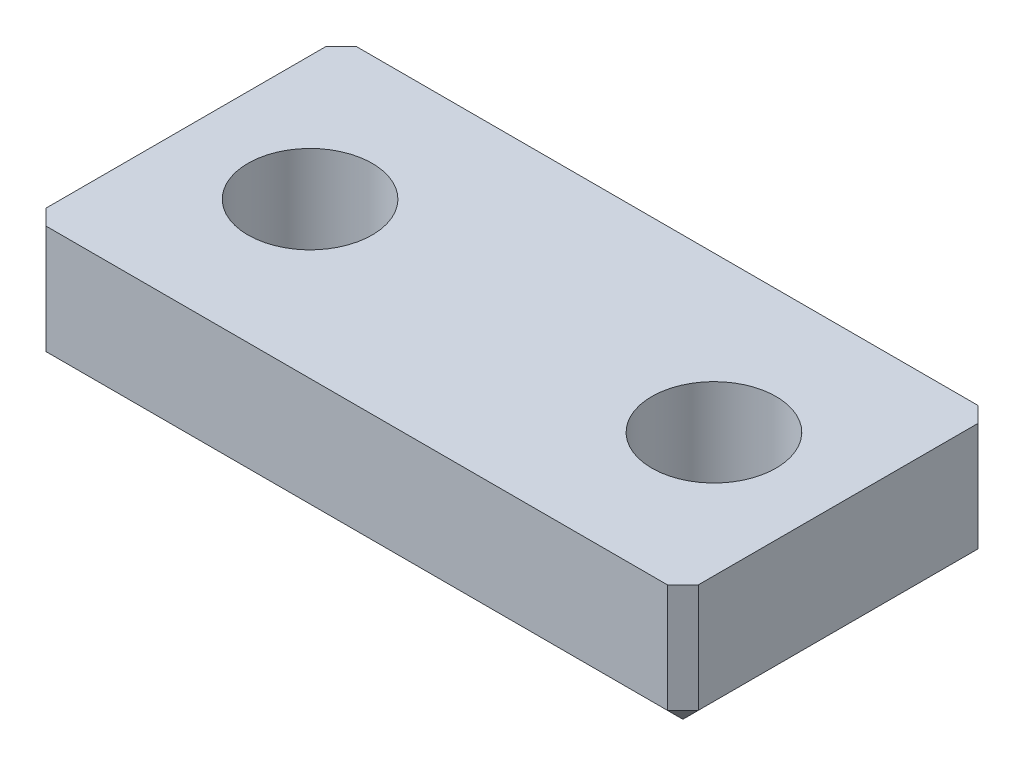
SolidWorks part; units mm, degrees
ref_plane "Front Plane" through (0, 0, 0) normal (0, 0, 1) x (1, 0, 0)
ref_plane "Top Plane" through (0, 0, 0) normal (0, 1, 0) x (1, 0, 0)
ref_plane "Right Plane" through (0, 0, 0) normal (1, 0, 0) x (0, 0, -1)
sketch "Sketch1" plane through (0, 0, 0) normal (0, 0, 1) x (1, 0, 0)
  line L1 (0, 0) -> (21, 0)
  line L2 (0, 0) -> (0, -4)
  line L3 (0, -4) -> (21, -4)
  line L4 (21, 0) -> (21, -4)
  dimension "D1" = 21
  dimension "D2" = 4
extrude "Boss-Extrude1" add sketch "Sketch1" along normal blind 10
sketch "Sketch2" plane through (0, 0, 0) normal (0, 1, 0) x (1, 0, 0)
  line L0 (21, -10) -> (21, 0) construction
  line L1 (0, -10) -> (0, 0) construction
  circle A0 centre (17, -5) radius 2
  circle A1 centre (4, -5) radius 2
  dimension "D1" = 4
  dimension "D2" = 4
  dimension "D3" = 4
  dimension "D4" = 4
extrude "Cut-Extrude1" cut sketch "Sketch2" against normal blind 10
chamfer "Chamfer2" distance 0.5 angle 45 12 edges at (21, -2, 0) (21, -2, 10) (0, -2, 0) (0, -2, 10) (21, 0, 5) (10.5, 0, 0) (0, 0, 5) (10.5, 0, 10) (0, -4, 5) (10.5, -4, 0) (21, -4, 5) (10.5, -4, 10)
